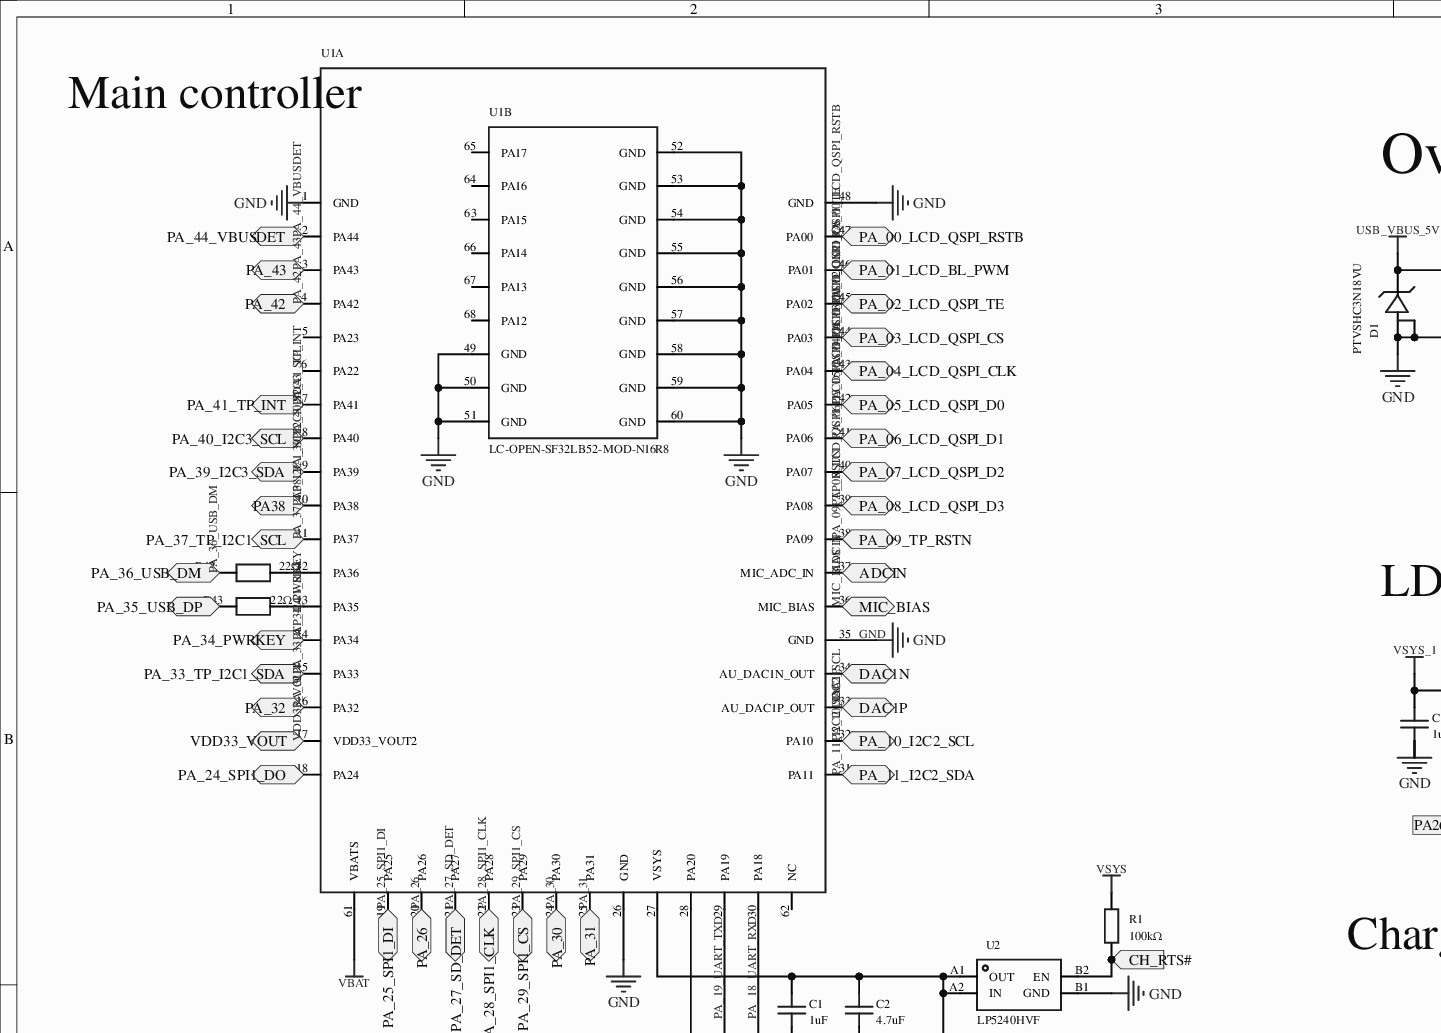
[diagram p0: MISC52032-3.schdoc, top left]
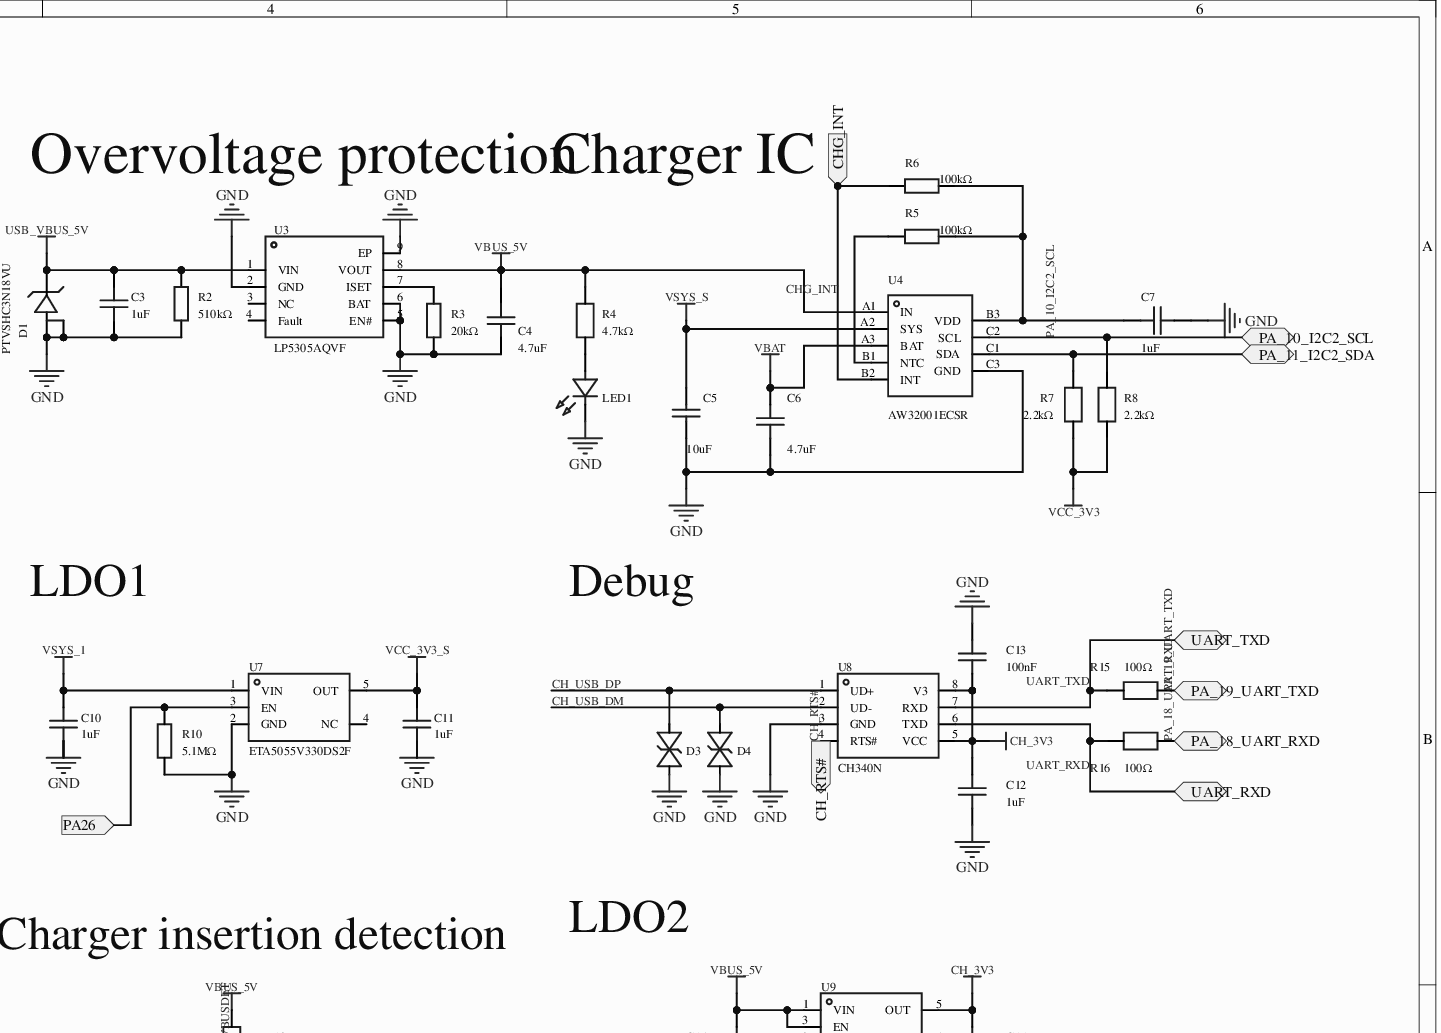
[diagram p1: MISC52032-3.schdoc, top right]
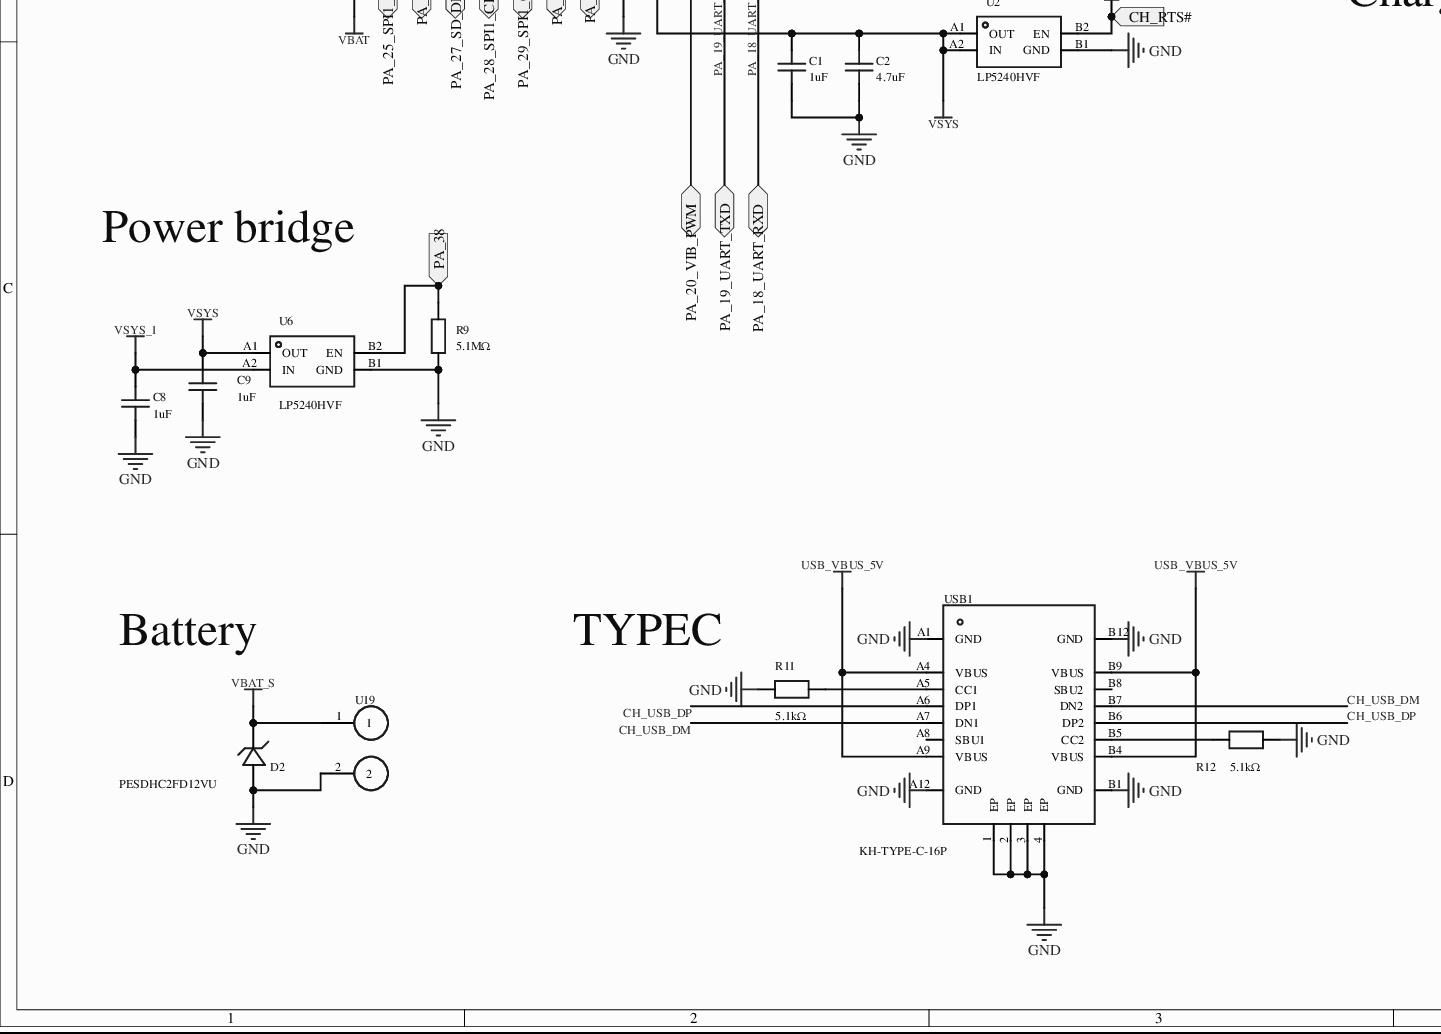
[diagram p2: MISC52032-3.schdoc, bottom left]
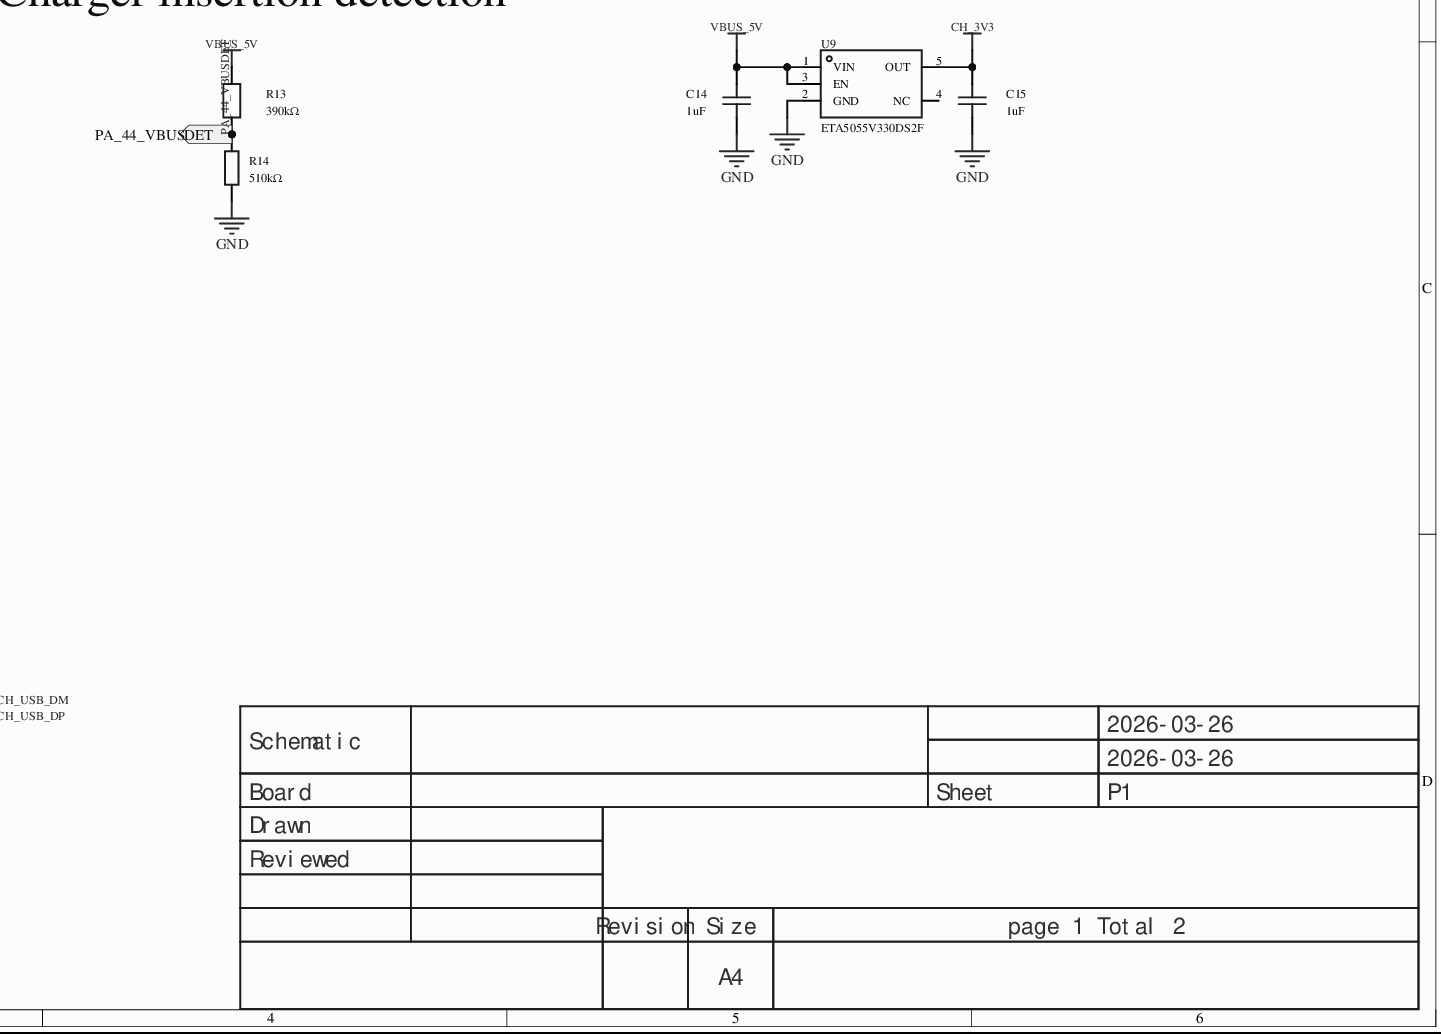
[diagram p3: MISC52032-3.schdoc, bottom right]
# Altium project MISC52032-2.PrjPcb (part 1 of 2)
2 sheets, 138 parts. Net scope: flat (ports and power ports of the same name join across sheets).
Board file: MISC52032.pcbdoc
Sheets:
  MISC52032-3.schdoc
  MISC52032-4.schdoc

## Sheet MISC52032-3.schdoc
size 420 x 297 mm; Version: V1.0; @Project Name: MISC52032; @Page Count: 2; @Update Date: 2026-03-26; @Create Date: 2026-03-26; @Schematic Name: MISC52032; @Page No: 1; @Board Name: MISC52032; @Create Time: 20:44:44; @Update Time: 20:59:57; Size: A4

### Parts
C1  1uF  [C0402]
C2  4.7uF  [C0402]
C3  1uF  [C0402]
C4  4.7uF  [C0402]
C5  10uF  [C0402]
C6  4.7uF  [C0402]
C7  1uF  [C0402]
C8  1uF  [C0402]
C9  1uF  [C0402]
C10  1uF  [C0402]
C11  1uF  [C0402]
C12  1uF  [C0402]
C13  100nF  [C0402]
C14  1uF  [C0402]
C15  1uF  [C0402]
D1  PTVSHC3N18VU  [DFN-3_L2.0-W2.0-P1.30-BR]
D2  PESDHC2FD12VU  [DFN1006-2L-RD]
D3  (no value)  [D0402-BI]
D4  (no value)  [D0402-BI]
LED1  (no value)  [LED0603-RD_GREEN]
R1  100kΩ  [R0402]
R2  510kΩ  [R0402]
R3  20kΩ  [R0402]
R4  4.7kΩ  [R0402]
R5  100kΩ  [R0402]
R6  100kΩ  [R0402]
R7  2.2kΩ  [R0402]
R8  2.2kΩ  [R0402]
R9  5.1MΩ  [R0402]
R10  5.1MΩ  [R0402]
R11  5.1kΩ  [R0402]
R12  5.1kΩ  [R0402]
R13  390kΩ  [R0402]
R14  510kΩ  [R0402]
R15  100Ω  [R0402]
R16  100Ω  [R0402]
R42  22Ω  [R0402]
R43  22Ω  [R0402]
U1  (no value)  [COMM-SMD_L27.9-W18.0-P1.10_SF32LB52-MOD-1-N16R8]  (parts A,B of 2)
U2  LP5240HVF  [WLCSP-4_L0.8-W0.8-R2-C2-P0.40-BL]
U3  LP5305AQVF  [DFN-8_L2.0-W2.0-P0.50-BL-EP]
U4  AW32001ECSR  [WLCSP-9_L1.7-W1.7-R3-C3-P0.50-TL]
U6  LP5240HVF  [WLCSP-4_L0.8-W0.8-R2-C2-P0.40-BL]
U7  ETA5055V330DS2F  [SOT-23-5_L2.9-W1.6-P0.95-LS2.8-BR]
U8  CH340N  [SOP-8_L4.9-W3.9-P1.27-LS6.0-BL]
U9  ETA5055V330DS2F  [SOT-23-5_L2.9-W1.6-P0.95-LS2.8-BR]
U19  (no value)  [焊盘]
USB1  KH-TYPE-C-16P  [USB-C-SMD_KH-TYPE-C-16P]

### Ports
ADCIN (bidir), CH_RTS# (in), CH_RTS# (out), CHG_INT (in), DAC1N (bidir), DAC1P (bidir), MIC_BIAS (bidir), PA26 (in), PA38 (bidir), PA_00_LCD_QSPI_RSTB (bidir), PA_01_LCD_BL_PWM (bidir), PA_02_LCD_QSPI_TE (bidir), PA_03_LCD_QSPI_CS (bidir), PA_04_LCD_QSPI_CLK (bidir), PA_05_LCD_QSPI_D0 (bidir), PA_06_LCD_QSPI_D1 (bidir), PA_07_LCD_QSPI_D2 (bidir), PA_08_LCD_QSPI_D3 (bidir), PA_09_TP_RSTN (bidir), PA_10_I2C2_SCL (bidir), PA_11_I2C2_SDA (bidir), PA_18_UART_RXD (bidir), PA_19_UART_TXD (bidir), PA_20_VIB_PWM (bidir), PA_24_SPI1_DO (bidir), PA_25_SPI1_DI (bidir), PA_26 (bidir), PA_27_SD_DET (bidir), PA_28_SPI1_CLK (bidir), PA_29_SPI1_CS (bidir), PA_30 (bidir), PA_31 (bidir), PA_32 (bidir), PA_33_TP_I2C1_SDA (bidir), PA_34_PWRKEY (bidir), PA_35_USB_DP (bidir), PA_36_USB_DM (bidir), PA_37_TP_I2C1_SCL (bidir), PA_38 (in), PA_39_I2C3_SDA (bidir), PA_40_I2C3_SCL (bidir), PA_41_TP_INT (bidir), PA_42 (bidir), PA_43 (bidir), PA_44_VBUSDET (bidir), PA_44_VBUSDET (out), UART_RXD (bidir), UART_TXD (bidir), VDD33_VOUT (bidir)

### Nets
CH_3V3: C12.2 C13.1 C15.2 U8.5(VCC) U8.8(V3) U9.5(OUT)
GND: C1.1 C2.1 C3.1 C4.1 C5.2 C6.2 C7.2 C8.1 C9.1 C10.1 C11.1 C12.1 C13.2 C14.1 C15.1 D1.1(A) D1.2(A) D2.2(A) D3.1(K) D4.1(K) LED1.1(C) R2.1 R3.1 R9.1 R10.1 R11.1 R12.2 R14.1 U1.1(GND) U1.26(GND) U1.35(GND) U1.48(GND) U1.49(GND) U1.50(GND) U1.51(GND) U1.52(GND) U1.53(GND) U1.54(GND) U1.55(GND) U1.56(GND) U1.57(GND) U1.58(GND) U1.59(GND) U1.60(GND) U2.B1(GND) U3.2(GND) U3.5(EN#) U3.6(BAT) U3.9(EP) U4.C3(GND) U6.B1(GND) U7.2(GND) U8.3(GND) U9.2(GND) U19.2 USB1.1(EP) USB1.2(EP) USB1.3(EP) USB1.4(EP) USB1.A1(GND) USB1.A12(GND) USB1.B1(GND) USB1.B12(GND)
USB_VBUS_5V: C3.2 D1.3(K) R2.2 U3.1(VIN) USB1.A4(VBUS) USB1.A9(VBUS) USB1.B4(VBUS) USB1.B9(VBUS)
VBAT: C6.1 U1.61(VBATS) U4.A3(BAT)
VBAT_S: D2.1(C) U19.1
VBUS_5V: C4.2 C14.2 R4.2 R13.2 U3.8(VOUT) U4.A1(IN) U9.1(VIN) U9.3(EN)
VCC_3V3: R7.1 R8.1
VCC_3V3_S: C11.2 U7.5(OUT)
VDD33_VOUT: U1.17(VDD33_VOUT2) ; port VDD33_VOUT
VSYS: C1.2 C2.2 C9.2 R1.2 U1.27(VSYS) U2.A1(OUT) U2.A2(IN) U6.A1(OUT)
VSYS_1: C8.2 C10.2 U6.A2(IN) U7.1(VIN)
VSYS_S: C5.1 U4.A2(SYS)
ADCIN: U1.37(MIC_ADC_IN) ; port ADCIN
CH_RTS#: R1.1 U2.B2(EN) U8.4(RTS#) ; port CH_RTS#
CH_USB_DM: D4.2(A) U8.2(UD-) USB1.A7(DN1) USB1.B7(DN2)
CH_USB_DP: D3.2(A) U8.1(UD+) USB1.A6(DP1) USB1.B6(DP2)
CHG_INT: R6.2 U4.B2(INT) ; port CHG_INT
DAC1N: U1.34(AU_DAC1N_OUT) ; port DAC1N
DAC1P: U1.33(AU_DAC1P_OUT) ; port DAC1P
MIC_BIAS: U1.36(MIC_BIAS) ; port MIC_BIAS
PA38: U1.10(PA38) ; port PA38
PA_00_LCD_QSPI_RSTB: U1.47(PA00) ; port PA_00_LCD_QSPI_RSTB
PA_01_LCD_BL_PWM: U1.46(PA01) ; port PA_01_LCD_BL_PWM
PA_02_LCD_QSPI_TE: U1.45(PA02) ; port PA_02_LCD_QSPI_TE
PA_03_LCD_QSPI_CS: U1.44(PA03) ; port PA_03_LCD_QSPI_CS
PA_04_LCD_QSPI_CLK: U1.43(PA04) ; port PA_04_LCD_QSPI_CLK
PA_05_LCD_QSPI_D0: U1.42(PA05) ; port PA_05_LCD_QSPI_D0
PA_06_LCD_QSPI_D1: U1.41(PA06) ; port PA_06_LCD_QSPI_D1
PA_07_LCD_QSPI_D2: U1.40(PA07) ; port PA_07_LCD_QSPI_D2
PA_08_LCD_QSPI_D3: U1.39(PA08) ; port PA_08_LCD_QSPI_D3
PA_09_TP_RSTN: U1.38(PA09) ; port PA_09_TP_RSTN
PA_10_I2C2_SCL: R8.2 U1.32(PA10) U4.C2(SCL) ; port PA_10_I2C2_SCL
PA_11_I2C2_SDA: R7.2 U1.31(PA11) U4.C1(SDA) ; port PA_11_I2C2_SDA
PA_18_UART_RXD: R16.2 U1.30(PA18) ; port PA_18_UART_RXD
PA_19_UART_TXD: R15.2 U1.29(PA19) ; port PA_19_UART_TXD
PA_20_VIB_PWM: U1.28(PA20) ; port PA_20_VIB_PWM
PA_25_SPI1_DI: U1.19(PA25) ; port PA_25_SPI1_DI
PA_26: U1.20(PA26) ; port PA_26
PA_27_SD_DET: U1.21(PA27) ; port PA_27_SD_DET
PA_28_SPI1_CLK: U1.22(PA28) ; port PA_28_SPI1_CLK
PA_29_SPI1_CS: U1.23(PA29) ; port PA_29_SPI1_CS
PA_30: U1.24(PA30) ; port PA_30
PA_31: U1.25(PA31) ; port PA_31
PA_32: U1.16(PA32) ; port PA_32
PA_33_TP_I2C1_SDA: U1.15(PA33) ; port PA_33_TP_I2C1_SDA
PA_34_PWRKEY: U1.14(PA34) ; port PA_34_PWRKEY
PA_35_USB_DP: R43.2 ; port PA_35_USB_DP
PA_36_USB_DM: R42.1 ; port PA_36_USB_DM
PA_37_TP_I2C1_SCL: U1.11(PA37) ; port PA_37_TP_I2C1_SCL
PA_39_I2C3_SDA: U1.9(PA39) ; port PA_39_I2C3_SDA
PA_40_I2C3_SCL: U1.8(PA40) ; port PA_40_I2C3_SCL
PA_41_TP_INT: U1.7(PA41) ; port PA_41_TP_INT
PA_42: U1.4(PA42) ; port PA_42
PA_43: U1.3(PA43) ; port PA_43
PA_44_VBUSDET: R13.1 R14.2 U1.2(PA44) ; port PA_44_VBUSDET
UART_RXD: R16.1 U8.6(TXD) ; port UART_RXD
UART_TXD: R15.1 U8.7(RXD) ; port UART_TXD
NetC7_1: C7.1 R5.1 R6.1 U4.B3(VDD)
NetLED1_2: LED1.2(A) R4.1
NetR3_2: R3.2 U3.7(ISET)
NetR5_2: R5.2 U4.B1(NTC)
NetR9_2: R9.2 U6.B2(EN) ; port PA_38
NetR10_2: R10.2 U7.3(EN) ; port PA26
NetR11_2: R11.2 USB1.A5(CC1)
NetR12_1: R12.1 USB1.B5(CC2)
NetR25_1: U1.18(PA24) ; port PA_24_SPI1_DO
NetR42_2: R42.2 U1.12(PA36)
NetR43_1: R43.1 U1.13(PA35)

Not connected (* = marked no-connect by the designer): U1 5(PA23)* 6(PA22)* 62(NC)* 63(PA15)* 64(PA16)* 65(PA17)* 66(PA14)* 67(PA13)* 68(PA12)*; U3 3(NC)* 4(Fault)*; U7 4(NC)*; U9 4(NC)*; USB1 A8(SBU1)* B8(SBU2)*

### Notes on the sheet
- Main controller
- Overvoltage protection
- Charger IC
- LDO1
- Debug
- Charger insertion detection
- LDO2
- Power bridge
- Battery
- TYPEC
- 2026-03-26
- Schematic
- Board
- Sheet
- P1
- Drawn
- Reviewed
- Revision
- Size
- A4
- page 1 Total 2

### Library data of the parts
C1 C3 C7-C12 C14 C15 = CL05A105KA5NQNC: Capacitance:1uF;Tolerance:±10%;Rated voltage:25V;Temperature coefficient:X5R;; Manufacturer: SAMSUNG(三星); AddInBom: yes; ModelId: 36a51122f27c49738f86b3bfa98863e0; ModelName: C0402_L1.0-W0.5-H0.5; ModelTransform: 39.37,19.685,0,0,0,0,0,0,0; Tolerance: ±10%; Voltage Rating: 25V; Temperature Coefficient: X5R; Symbol: CL05A105KA5NQNC; Device: CL05A105KA5NQNC; LCSC Part Name: 1uF ±10% 25V; SupplierPart: C52923; ManufacturerPart: CL05A105KA5NQNC; Supplier Footprint: 0402; JLCPCB Part Class: Basic library; Datasheet: example.com/datasheet/CL05A105KA5NQNC/53938.html; Supplier: LCSC; ConvertToPcb: yes; FootprintName: C0402; Value: 1uF
C2 C4 C6 = CL05A475MP5NRNC: Capacitance:4.7uF;Tolerance:±20%;Rated voltage:10V;Temperature coefficient:X5R;; Manufacturer: SAMSUNG(三星); AddInBom: yes; ModelId: 36a51122f27c49738f86b3bfa98863e0; ModelName: C0402_L1.0-W0.5-H0.5; ModelTransform: 39.37,19.685,0,0,0,0,0,0,0; Tolerance: ±20%; Voltage Rating: 10V; Temperature Coefficient: X5R; Symbol: CL05A475MP5NRNC; Device: CL05A475MP5NRNC; LCSC Part Name: 4.7uF ±20% 10V; SupplierPart: C23733; ManufacturerPart: CL05A475MP5NRNC; Supplier Footprint: 0402; JLCPCB Part Class: Basic library; Datasheet: example.com/datasheet/CL05A475MP5NRNC/24469.html; Supplier: LCSC; ConvertToPcb: yes; FootprintName: C0402; Value: 4.7uF
C5 = CL05A106MQ5NUNC: Capacitance:10uF;Tolerance:±20%;Rated voltage:6.3V;Temperature coefficient:X5R;; Manufacturer: SAMSUNG(三星); AddInBom: yes; ModelId: 36a51122f27c49738f86b3bfa98863e0; ModelName: C0402_L1.0-W0.5-H0.5; ModelTransform: 39.37,19.685,0,0,0,0,0,0,0; Tolerance: ±20%; Voltage Rating: 6.3V; Temperature Coefficient: X5R; Symbol: CL05A106MQ5NUNC; Device: CL05A106MQ5NUNC; LCSC Part Name: 10uF ±20% 6.3V; SupplierPart: C15525; ManufacturerPart: CL05A106MQ5NUNC; Supplier Footprint: 0402; JLCPCB Part Class: Basic library; Datasheet: example.com/datasheet/CL05A106MQ5NUNC/16204.html; Supplier: LCSC; ConvertToPcb: yes; FootprintName: C0402; Value: 10uF
C13 = CL05B104KO5NNNC: Capacitance:100nF;Tolerance:±10%;Rated voltage:16V;Temperature coefficient:X7R;; Manufacturer: SAMSUNG(三星); AddInBom: yes; ModelId: 36a51122f27c49738f86b3bfa98863e0; ModelName: C0402_L1.0-W0.5-H0.5; ModelTransform: 39.37,19.685,0,0,0,0,0,0,0; Tolerance: ±10%; Voltage Rating: 16V; Temperature Coefficient: X7R; Symbol: CL05B104KO5NNNC; Device: CL05B104KO5NNNC; LCSC Part Name: 100nF ±10% 16V; SupplierPart: C1525; ManufacturerPart: CL05B104KO5NNNC; Supplier Footprint: 0402; JLCPCB Part Class: Basic library; Datasheet: example.com/datasheet/CL05B104KO5NNNC/1877.html; Supplier: LCSC; ConvertToPcb: yes; FootprintName: C0402; Value: 100nF
D1 = PTVSHC3N18VU: Reverse standoff voltage (Vrwm):18V;Clamping voltage:33V;Peak pulse current (Ipp):138A@8/20us;Peak pulse power (Ppp):4kW@8/20us;Breakdown voltage:20V;; Manufacturer: Prisemi(芯导); AddInBom: yes; ModelId: 63242cc9aa954e8686236999c1a1184a; ModelName: DFN-3_L2.0-W2.0-H0.6-P1.30-BR; ModelTransform: 79.527,79.527,0,90,0,0,-8.858,0,0; Reverse Stand-Off Voltage (Vrwm): 18V; Clamping Voltage: 33V; Voltage - Breakdown: 20V; Reverse Leakage Current (Ir): 1uA; Number of Channels: Single channel; level of protection: IEC 61000-4-4;IEC 61000-4-5;IEC 61000-4-2; Type: TVS; Junction Capacitance: 900pF; Symbol: PTVSHC3N18VU; Device: PTVSHC3N18VU; LCSC Part Name: TVS 18V截止 峰值脉冲电流：138A@8/20us; SupplierPart: C312227; ManufacturerPart: PTVSHC3N18VU; Supplier Footprint: DFN2x2-3L; JLCPCB Part Class: Extended library; Datasheet: example.com/datasheet/PTVSHC3N18VU/295148.html; Supplier: LCSC; ConvertToPcb: yes; FootprintName: DFN-3_L2.0-W2.0-P1.30-BR; Peak Pulse Current (Ipp): 138A@8/20us; Peak Pulse Power Dissipation (Ppp): 4kW@8/20us
D2 = PESDHC2FD12VU: Manufacturer: Prisemi(芯导); AddInBom: yes; ModelId: 96b2cca1435e47b08b55ab6e73617580; ModelName: DFN1006_L1-W0.6-H0.4-2L-RD; ModelTransform: 40.1574,24.4094,0,0,0,0,0,0,0; Symbol: PESDHC2FD12VU; Device: PESDHC2FD12VU; LCSC Part Name: PESDHC2FD12VU; SupplierPart: C496537; ManufacturerPart: PESDHC2FD12VU; Supplier Footprint: DFN1006-2L; JLCPCB Part Class: Extended library; Datasheet: example.com/upload/public/pdf/source/20200316/C496537_D4D5EFB16D45800B48AEB35AB1FE765F.pdf; Supplier: LCSC; ConvertToPcb: yes; FootprintName: DFN1006-2L-RD
D3 D4 = KLXES15AAA1: Polarity:Bidirectional;Reverse standoff voltage (Vrwm):5V;Clamping voltage:40V;Peak pulse current (Ipp):-;Peak pulse power (Ppp):-;Breakdown voltage:-;; Manufacturer: KUU; AddInBom: yes; ModelId: 62a80a189f1b46df8ba79817b730b378; ModelName: D0402_L1.0-W0.5-H0.5; ModelTransform: 39.37,19.685,0,0,0,0,0,0,0; Reverse Stand-Off Voltage (Vrwm): 5V; Clamping Voltage: 40V; Reverse Leakage Current (Ir): 10nA; Number of Channels: Single channel; level of protection: IEC 61000-4-2; Type: ESD; Junction Capacitance: 0.05pF; Symbol: KLXES15AAA1; Device: KLXES15AAA1; LCSC Part Name: 双向ESD 5V截止; SupplierPart: C2892490; Supplier Footprint: 0402; JLCPCB Part Class: Extended library; Datasheet: example.com/datasheet/KLXES15AAA1/3124109.html; Supplier: LCSC; ConvertToPcb: yes; FootprintName: D0402-BI; Polarity: Bidirectional; Peak Pulse Current (Ipp): -; Peak Pulse Power Dissipation (Ppp): -; Voltage - Breakdown: -; Operating Temperature: -55℃~+125℃
LED1 = F.0603.00025/P2-0603G1TS2-06T-002: Lamp type:-;Emitted color:Emerald green;Forward voltage (Vf):2.6V~2.9V;Power:90mW;Forward current:30mA;Wavelength:520nm~525nm;Diode configuration:Discrete diode;Lens color:-;Color temperature:-;Luminous intensity:230mcd;Viewing angle:120°;Tape and reel:-;Operating temperature:-40℃~+85℃;; Manufacturer: TUOZHAN(拓展光电); AddInBom: yes; ModelId: 7761174b67d9475ab0dbce38062fb2f9; ModelTransform: 63.7794,31.496,0,0,0,0,0,0,0; Power(Watts): 90mW; Forward Current: 30mA; Peak Wavelength: 517nm; Luminous Intensity: 230mcd; Viewing Angle: 120°; Symbol: F.0603.00025/P2-0603G1TS2-06T-002; Device: F.0603.00025/P2-0603G1TS2-06T-002; LCSC Part Name: 0603翠绿; SupplierPart: C7496818; Supplier Footprint: 0603; JLCPCB Part Class: Extended library; Datasheet: example.com/datasheet/F.0603.00025%252FP2-0603G1TS2-06T-002/8563182.html; Supplier: LCSC; ConvertToPcb: yes; FootprintName: LED0603-RD_GREEN; ModelName: LED0603-RD_GREEN; Lamp Holder Type: -; Illumination Color: Emerald green; Voltage - Forward(Vf): 2.6V~2.9V; Wavelength - Dominant: 520nm~525nm; Diode Configuration: Discrete diode; Lens Color: -; Color Temperature: -; Mounting Style: -; Operating Temperature: -40℃~+85℃
R1 R5 R6 = 0402WGF1003TCE: Resistor type:Thick-film resistor;Resistance:100kΩ;Tolerance:±1%;Power:62.5mW;Operating voltage:50V;Temperature coefficient:±100ppm/℃;; Manufacturer: UNI-ROYAL(厚声); AddInBom: yes; ModelId: 98c88bc2b9094f218f3a3e30a7012738; ModelName: R0402_L1.0-W0.5-H0.4; ModelTransform: 39.37,19.685,0,0,0,0,0,0,0; Tolerance: ±1%; Power(Watts): 62.5mW; Voltage-Supply(Max): 50V; Symbol: 0402WGF1003TCE; Device: 0402WGF1003TCE; LCSC Part Name: 100kΩ ±1% 62.5mW 厚膜电阻; SupplierPart: C25741; ManufacturerPart: 0402WGF1003TCE; Supplier Footprint: 0402; JLCPCB Part Class: Basic library; Datasheet: example.com/datasheet/0402WGF1003TCE/26484.html; Supplier: LCSC; ConvertToPcb: yes; FootprintName: R0402; Type: Thick-film resistor; Value: 100kΩ; Temperature Coefficient: ±100ppm/℃; Operating Temperature: -55℃~+155℃
R2 R14 = 0402WGF5103TCE: Resistor type:Thick-film resistor;Resistance:510kΩ;Tolerance:±1%;Power:62.5mW;Operating voltage:50V;Temperature coefficient:±100ppm/℃;; Manufacturer: UNI-ROYAL(厚声); AddInBom: yes; ModelId: 98c88bc2b9094f218f3a3e30a7012738; ModelName: R0402_L1.0-W0.5-H0.4; ModelTransform: 39.37,19.685,0,0,0,0,0,0,0; Tolerance: ±1%; Power(Watts): 62.5mW; Voltage-Supply(Max): 50V; Symbol: 0402WGF5103TCE; Device: 0402WGF5103TCE; LCSC Part Name: 510kΩ ±1% 62.5mW 厚膜电阻; SupplierPart: C11616; ManufacturerPart: 0402WGF5103TCE; Supplier Footprint: 0402; JLCPCB Part Class: Extended library; Datasheet: example.com/datasheet/0402WGF5103TCE/12170.html; Supplier: LCSC; ConvertToPcb: yes; FootprintName: R0402; Type: Thick-film resistor; Value: 510kΩ; Temperature Coefficient: ±100ppm/℃; Operating Temperature: -55℃~+155℃
R3 = FRC0402F2002TS: Resistor type:Thick-film resistor;Resistance:20kΩ;Tolerance:±1%;Power:62.5mW;Operating voltage:50V;Temperature coefficient:±100ppm/℃;; Manufacturer: FOJAN(富捷); AddInBom: yes; ModelId: 98c88bc2b9094f218f3a3e30a7012738; ModelName: R0402_L1.0-W0.5-H0.4; ModelTransform: 39.37,19.685,0,0,0,0,0,0,0; Tolerance: ±1%; Power(Watts): 62.5mW; Voltage-Supply(Max): 50V; Symbol: FRC0402F2002TS; Device: FRC0402F2002TS; LCSC Part Name: 20kΩ ±1% 62.5mW 厚膜电阻; SupplierPart: C2906867; ManufacturerPart: FRC0402F2002TS; Supplier Footprint: 0402; JLCPCB Part Class: Extended library; Datasheet: example.com/datasheet/FRC0402F2002TS/3180380.html; Supplier: LCSC; ConvertToPcb: yes; FootprintName: R0402; Type: Thick-film resistor; Value: 20kΩ; Temperature Coefficient: ±100ppm/℃; Operating Temperature: -55℃~+155℃
R4 = FRC0402F4701TS: Resistor type:Thick-film resistor;Resistance:4.7kΩ;Tolerance:±1%;Power:62.5mW;Operating voltage:50V;Temperature coefficient:±100ppm/℃;; Manufacturer: FOJAN(富捷); AddInBom: yes; ModelId: 98c88bc2b9094f218f3a3e30a7012738; ModelName: R0402_L1.0-W0.5-H0.4; ModelTransform: 39.37,19.685,0,0,0,0,0,0,0; Tolerance: ±1%; Power(Watts): 62.5mW; Voltage-Supply(Max): 50V; Symbol: FRC0402F4701TS; Device: FRC0402F4701TS; LCSC Part Name: 4.7kΩ ±1% 62.5mW 厚膜电阻; SupplierPart: C2906869; ManufacturerPart: FRC0402F4701TS; Supplier Footprint: 0402; JLCPCB Part Class: Extended library; Supplier: LCSC; ConvertToPcb: yes; FootprintName: R0402; Type: Thick-film resistor; Value: 4.7kΩ; Temperature Coefficient: ±100ppm/℃; Operating Temperature: -55℃~+155℃
R7 R8 = FRC0402F2201TS: Resistor type:Thick-film resistor;Resistance:2.2kΩ;Tolerance:±1%;Power:62.5mW;Operating voltage:50V;Temperature coefficient:±100ppm/℃;; Manufacturer: FOJAN(富捷); AddInBom: yes; ModelId: 98c88bc2b9094f218f3a3e30a7012738; ModelName: R0402_L1.0-W0.5-H0.4; ModelTransform: 39.37,19.685,0,0,0,0,0,0,0; Tolerance: ±1%; Power(Watts): 62.5mW; Voltage-Supply(Max): 50V; Symbol: FRC0402F2201TS; Device: FRC0402F2201TS; LCSC Part Name: 2.2kΩ ±1% 62.5mW 厚膜电阻; SupplierPart: C2906865; ManufacturerPart: FRC0402F2201TS; Supplier Footprint: 0402; JLCPCB Part Class: Extended library; Datasheet: example.com/datasheet/FRC0402F2201TS/3180378.html; Supplier: LCSC; ConvertToPcb: yes; FootprintName: R0402; Type: Thick-film resistor; Value: 2.2kΩ; Temperature Coefficient: ±100ppm/℃; Operating Temperature: -55℃~+155℃
R9 R10 = 0402WGF5104TCE: Resistor type:Thick-film resistor;Resistance:5.1MΩ;Tolerance:±1%;Power:62.5mW;Operating voltage:50V;Temperature coefficient:±100ppm/℃;; Manufacturer: UNI-ROYAL(厚声); AddInBom: yes; ModelId: 98c88bc2b9094f218f3a3e30a7012738; ModelName: R0402_L1.0-W0.5-H0.4; ModelTransform: 39.37,19.685,0,0,0,0,0,0,0; Tolerance: ±1%; Power(Watts): 62.5mW; Voltage-Supply(Max): 50V; Symbol: 0402WGF5104TCE; Device: 0402WGF5104TCE; LCSC Part Name: 5.1MΩ ±1% 62.5mW 厚膜电阻; SupplierPart: C270595; ManufacturerPart: 0402WGF5104TCE; Supplier Footprint: 0402; JLCPCB Part Class: Extended library; Datasheet: example.com/datasheet/0402WGF5104TCE/259975.html; Supplier: LCSC; ConvertToPcb: yes; FootprintName: R0402; Type: Thick-film resistor; Value: 5.1MΩ; Temperature Coefficient: ±100ppm/℃; Operating Temperature: -55℃~+155℃
R11 R12 = FRC0402F5101TS: Resistor type:Thick-film resistor;Resistance:5.1kΩ;Tolerance:±1%;Power:62.5mW;Operating voltage:50V;Temperature coefficient:±100ppm/℃;; Manufacturer: FOJAN(富捷); AddInBom: yes; ModelId: 98c88bc2b9094f218f3a3e30a7012738; ModelName: R0402_L1.0-W0.5-H0.4; ModelTransform: 39.37,19.685,0,0,0,0,0,0,0; Tolerance: ±1%; Power(Watts): 62.5mW; Voltage-Supply(Max): 50V; Symbol: FRC0402F5101TS; Device: FRC0402F5101TS; LCSC Part Name: 5.1kΩ ±1% 62.5mW 厚膜电阻; SupplierPart: C2906874; ManufacturerPart: FRC0402F5101TS; Supplier Footprint: 0402; JLCPCB Part Class: Extended library; Supplier: LCSC; ConvertToPcb: yes; FootprintName: R0402; Type: Thick-film resistor; Value: 5.1kΩ; Temperature Coefficient: ±100ppm/℃; Operating Temperature: -55℃~+155℃
R13 = FRC0402F3903TS: Resistor type:Thick-film resistor;Resistance:390kΩ;Tolerance:±1%;Power:62.5mW;Operating voltage:50V;Temperature coefficient:±100ppm/℃;; Manufacturer: FOJAN(富捷); AddInBom: yes; ModelId: 98c88bc2b9094f218f3a3e30a7012738; ModelName: R0402_L1.0-W0.5-H0.4; ModelTransform: 39.37,19.685,0,0,0,0,0,0,0; Tolerance: ±1%; Power(Watts): 62.5mW; Voltage-Supply(Max): 50V; Symbol: FRC0402F3903TS; Device: FRC0402F3903TS; LCSC Part Name: 390kΩ ±1% 62.5mW 厚膜电阻; SupplierPart: C2909352; ManufacturerPart: FRC0402F3903TS; Supplier Footprint: 0402; JLCPCB Part Class: Extended library; Supplier: LCSC; ConvertToPcb: yes; FootprintName: R0402; Type: Thick-film resistor; Value: 390kΩ; Temperature Coefficient: ±100ppm/℃; Operating Temperature: -55℃~+155℃
R15 R16 = FRC0402F1000TS: Resistor type:Thick-film resistor;Resistance:100Ω;Tolerance:±1%;Power:62.5mW;Operating voltage:50V;Temperature coefficient:±100ppm/℃;; Manufacturer: FOJAN(富捷); AddInBom: yes; ModelId: 98c88bc2b9094f218f3a3e30a7012738; ModelName: R0402_L1.0-W0.5-H0.4; ModelTransform: 39.37,19.685,0,0,0,0,0,0,0; Tolerance: ±1%; Power(Watts): 62.5mW; Voltage-Supply(Max): 50V; Symbol: FRC0402F1000TS; Device: FRC0402F1000TS; LCSC Part Name: 100Ω ±1% 62.5mW 厚膜电阻; SupplierPart: C2906860; ManufacturerPart: FRC0402F1000TS; Supplier Footprint: 0402; JLCPCB Part Class: Extended library; Supplier: LCSC; ConvertToPcb: yes; FootprintName: R0402; Type: Thick-film resistor; Value: 100Ω; Temperature Coefficient: ±100ppm/℃; Operating Temperature: -55℃~+155℃
R42 R43 = FRC0402J220 TS: Resistor type:Thick-film resistor;Resistance:22Ω;Tolerance:±5%;Power:62.5mW;Operating voltage:50V;Temperature coefficient:±100ppm/℃;; Manufacturer: FOJAN(富捷); AddInBom: yes; ModelId: 98c88bc2b9094f218f3a3e30a7012738; ModelName: R0402_L1.0-W0.5-H0.4; ModelTransform: 39.37,19.685,0,0,0,0,0,0,0; Tolerance: ±5%; Power(Watts): 62.5mW; Voltage-Supply(Max): 50V; Symbol: FRC0402J220 TS; Device: FRC0402J220 TS; LCSC Part Name: 22Ω ±5% 62.5mW 厚膜电阻; SupplierPart: C2906914; ManufacturerPart: FRC0402J220 TS; Supplier Footprint: 0402; JLCPCB Part Class: Extended library; Datasheet: example.com/datasheet/FRC0402J220%2520TS/3180427.html; Supplier: LCSC; ConvertToPcb: yes; FootprintName: R0402; Type: Thick-film resistor; Value: 22Ω; Temperature Coefficient: ±100ppm/℃; Operating Temperature: -55℃~+155℃
U1 = LC-OPEN-SF32LB52-MOD-N16R8: Core chip:SF32LB525UC6 chip;Interface types:I2C; LCD; SPI; UART; USB; I2S; SDIO;Transmit power:19dBm;Communication distance:-;Receive sensitivity:-100dBm;; Manufacturer: 立创开发板; Symbol: SF32LB52-MOD-1-N16R8; Relevance: []; AddInBom: yes; ModelId: 92a4f358e48d41b0bab2544589b6c55b; ModelTransform: 708.73866,1098.46237,0,0,0,0,-0.001,131.457,0; Wireless Standard: Bluetooth 5.3; Output Power(Max): 19dBm; Voltage - Supply: 3.2V~4.7V; Antenna Type: On-board PCB antenna; Receive  Current: 2mA; Send  Current: 2.6mA; Device: LC-OPEN-SF32LB52-MOD-N16R8; LCSC Part Name: 立创·开源SF32LB52模组; SupplierPart: C42924267; Supplier Footprint: SMD,18x27.9mm; JLCPCB Part Class: Extended library; Supplier: LCSC; ConvertToPcb: yes; FootprintName: COMM-SMD_L27.9-W18.0-P1.10_SF32LB52-MOD-1-N16R8; ModelName: COMM-SMD_L27.9-W18.0-P1.10_SF32LB52-MOD-1-N16R8; Utilized IC / Part: SF32LB525UC6 chip; Interface Type: I2C; LCD; SPI; UART; USB; I2S; SDIO; Communication Distance: -; Sensitivity: -100dBm; Operating Temperature: -40℃~+85℃
U2 U6 = LP5240HVF: Type:Load switch;Channels:1;Input control logic:Active high;Max continuous current:1.5A;Operating voltage:1.2V~5.5V;On-resistance:50mΩ;; Manufacturer: LOWPOWER(微源半导体); AddInBom: yes; ModelId: fa444c8b39994a7a9c440f434d4dd0a4; ModelName: WLCSP-4_L0.8-W0.8-H0.6-P0.4; ModelTransform: 31.496,31.496,0,90,0,0,-0.005,0.003,0; Number of Channels: 1; Maximum Continuous Current: 1.5A; RDS(on): 50mΩ; Symbol: LP5240HVF; Device: LP5240HVF; LCSC Part Name: LP5240HVF; SupplierPart: C2890373; ManufacturerPart: LP5240HVF; Supplier Footprint: WLCSP-4; JLCPCB Part Class: Extended library; Datasheet: example.com/datasheet/LP5240HVF/3114301.html; Supplier: LCSC; ConvertToPcb: yes; FootprintName: WLCSP-4_L0.8-W0.8-R2-C2-P0.40-BL; Type: Load switch; Control Input Logic: Active high; Voltage - Supply: 1.2V~5.5V; Operating Temperature	-: -40℃~+85℃
U3 = LP5305AQVF: Operating voltage:3.3V~26V;Max charge current:1A;Battery type:Lithium battery;Number of cells:1;; Manufacturer: LOWPOWER(微源半导体); AddInBom: yes; ModelId: ea9fe5daec6c437ca860910abaae89ca; ModelName: DFN-8_L2.0-W2.0-H0.8-P0.50; ModelTransform: 78.74,77.961,0,90,0,0,0,0,0; The Chip Type: Protection chip; Charge Current - Max: 1A; Charging Saturation Voltage: 4.35V; Number of Cells: 1; Battery Temperature Detection: Not supported; Supply Current (Iq): 55uA; Symbol: LP5305AQVF; Device: LP5305AQVF; LCSC Part Name: 过压和过流保护集成电路; SupplierPart: C517045; ManufacturerPart: LP5305AQVF; Supplier Footprint: DFN-8-EP(2x2); JLCPCB Part Class: Extended library; Datasheet: example.com/datasheet/LP5305AQVF/533410.html; Supplier: LCSC; ConvertToPcb: yes; FootprintName: DFN-8_L2.0-W2.0-P0.50-BL-EP; Voltage - Supply: 3.3V~26V; End-Off Voltage: -; Type of Battery: Lithium battery; Operating Temperature: -40℃~+105℃; 0V Battery Charge: -; Balance Current: -; Interface: -
U4 = AW32001ECSR: Operating voltage:4V~5.5V;Max charge current:500mA;Battery type:Lithium battery;Number of cells:1;; Manufacturer: AWINIC(艾为); AddInBom: yes; ModelId: 57ce10a4838745eab5f0c477e6bbd013; ModelTransform: 64.961,73.6219,0,0,0,0,0,0,0; The Chip Type: Charging chip; Charge Current - Max: 500mA; Charging Saturation Voltage: 4.2V; Number of Cells: 1; Battery Temperature Detection: Supported; Supply Current (Iq): 1uA; Interface: I2C; Symbol: AW32001ECSR; Device: AW32001ECSR; LCSC Part Name: 单节锂离子电池充电器，具备电源路径管理和完全 USB 兼容性; SupplierPart: C5125890; ManufacturerPart: AW32001ECSR; Supplier Footprint: WLCSP-9-B(1.68x1.68); JLCPCB Part Class: Extended library; Datasheet: example.com/datasheet/AW32001ECSR/5725683.html; Supplier: LCSC; ConvertToPcb: yes; FootprintName: WLCSP-9_L1.7-W1.7-R3-C3-P0.50-TL; ModelName: WLCSP-9_L1.7-W1.7-R3-C3-P0.50-TL; Voltage - Supply: 4V~5.5V; End-Off Voltage: -; Type of Battery: Lithium battery; Operating Temperature: -40℃~+85℃; 0V Battery Charge: Supported; Balance Current: -
U7 U9 = ETA5055V330DS2F: Output type:Fixed;Operating voltage:5.5V;Output voltage:3.3V;Output current:500mA;Power supply rejection ratio (PSRR):94dB@(1kHz);Output polarity:Positive;; Manufacturer: ETA(钰泰); AddInBom: yes; ModelId: 7ba65df16e7b4570af156e925f9c37fe; ModelTransform: 114.173,114.173,0,90,0,0,0,0,0; Output Type: Fixed; Voltage - Supply: 5.5V; Output Voltage: 3.3V; Output Current: 500mA; Voltage Dropout: 90mV@(200mA); standby current: 4.5uA; Number of Outputs: 1; Symbol: ETA5055V330DS2F; Device: ETA5055V330DS2F; LCSC Part Name: 适用于射频和模拟电路的超高电源抑制比、超低静态电流、500mA低压差线性稳压器; SupplierPart: C22362747; ManufacturerPart: ETA5055V330DS2F; Supplier Footprint: SOT-23-5; JLCPCB Part Class: Extended library; Datasheet: example.com/datasheet/ETA5055V330DS2F/23810798.html; Supplier: LCSC; ConvertToPcb: yes; FootprintName: SOT-23-5_L2.9-W1.6-P0.95-LS2.8-BR; ModelName: SOT-23-5_L2.9-W1.6-P0.95-LS2.8-BR; Power Supply Rejection Ratio (PSRR): 94dB@(1kHz); Features: Overcurrent protection; enable; overtemperature protection; short-circuit protection; Operating Temperature: -40℃~+85℃@(Ta); Output Configuration: Positive
U8 = CH340N: Application function:USB to serial;USB version:USB 2.0;Channels:1;Data rate:2Mbps;; Manufacturer: WCH(南京沁恒); Symbol: CH340N_C2977777; AddInBom: yes; ModelId: 75c24a7891ee4dd6bdac16a7163ff87e; ModelName: SOP-8_L4.9-W3.9-P1.27-LS6.0-BL-1; ModelTransform: 192.913,236.22,0,0,0,0,0,0,0; USB Protocol: USB 2.0; Number of Channels: 1; Voltage - Supply: 3.3V; 5V; Data Rate: 2Mbps; Device: CH340N; LCSC Part Name: USB2.0芯片CH340; SupplierPart: C2977777; ManufacturerPart: CH340N; Supplier Footprint: SOP-8; JLCPCB Part Class: Extended library; Datasheet: example.com/datasheet/CH340N/3390257.html; Supplier: LCSC; ConvertToPcb: yes; FootprintName: SOP-8_L4.9-W3.9-P1.27-LS6.0-BL; Applications Function: USB to serial; Operating Temperature: -20℃~+70℃
U19 = 焊盘: Device: Pad; AddInBom: yes; ConvertToPcb: yes; SymbolName: Pad; FootprintName: Pad
USB1 = KH-TYPE-C-16P: Connector type:Type-C;Protocol standard:-;Gender:Female;Mounting:Horizontal;Number of contacts:16P;Number of ports:1;Rated current - power:3A;Operating temperature:-40℃~+85℃;; Manufacturer: kinghelm(金航标); AddInBom: yes; ModelId: f2c381012fbf47e0b76dea5162270f01; ModelTransform: 351.9678,307.48,0,0,0,0,0,-45.276,-43.307; Connector Type: Type-C; Gender: Female; Number of Contacts: 16P; Number of Ports: 1; Current Rating-Power: 3A; Voltage Rating: 30V; Connect-Disconnect Life: 1万 cycles; Symbol: KH-TYPE-C-16P; Device: KH-TYPE-C-16P; LCSC Part Name: Type-C 母 卧贴; SupplierPart: C709357; ManufacturerPart: KH-TYPE-C-16P; Supplier Footprint: SMD; JLCPCB Part Class: Extended library; Datasheet: example.com/datasheet/KH-TYPE-C-16P/747093.html; Supplier: LCSC; ConvertToPcb: yes; FootprintName: USB-C-SMD_KH-TYPE-C-16P; ModelName: USB-C-SMD_KH-TYPE-C-16P; Protocol Standard: -; Mounting Type: Horizontal mount; Length: 7.81mm; Operating Temperature: -40℃~+85℃